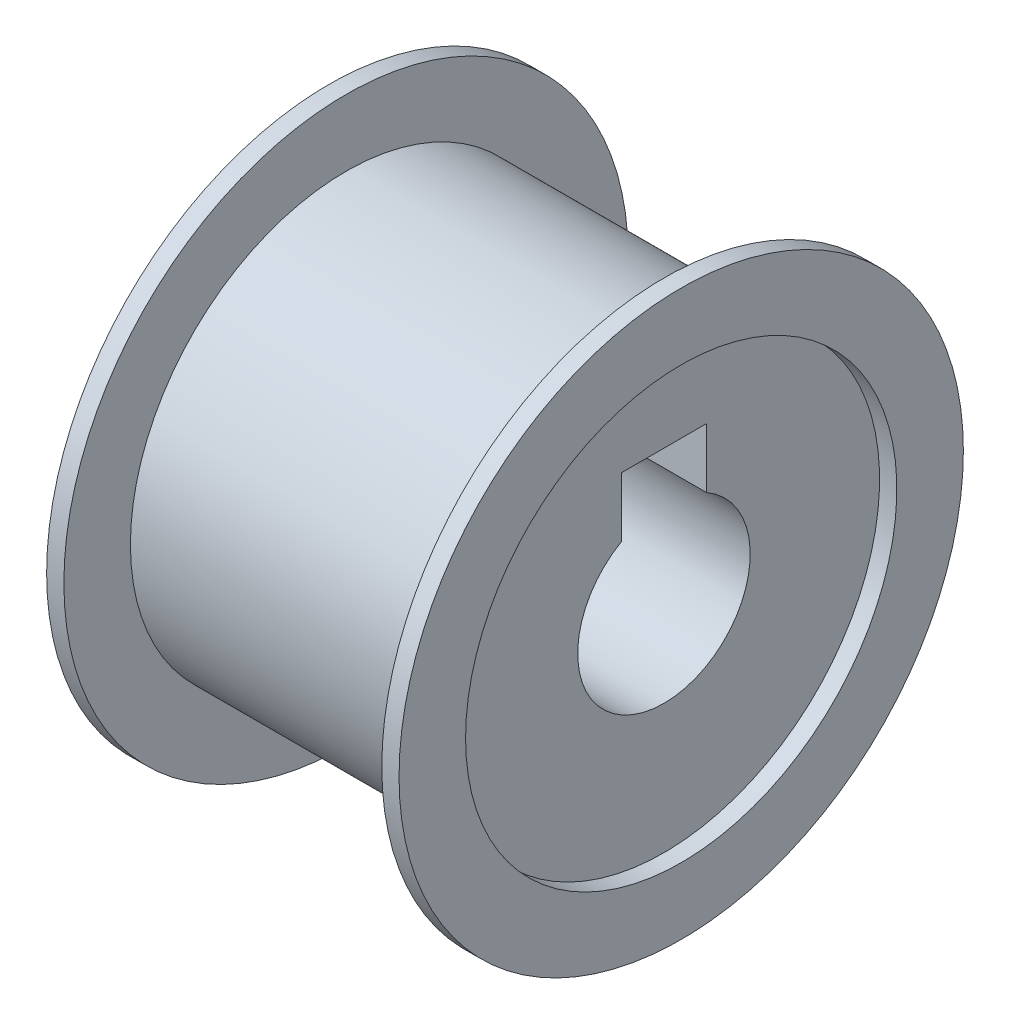
SolidWorks part; units mm, degrees
ref_plane "Front Plane" through (0, 0, 0) normal (0, 0, 1) x (1, 0, 0)
ref_plane "Top Plane" through (0, 0, 0) normal (0, 1, 0) x (1, 0, 0)
ref_plane "Right Plane" through (0, 0, 0) normal (1, 0, 0) x (0, 0, -1)
sketch "Sketch1" plane through (0, 0, 0) normal (0, 1, 0) x (1, 0, 0)
  line L0 (0, 0) -> (3.0534, 0) construction
  line L5 (-2.0429, 2.5) -> (2.0429, 2.5)
  line L6 (-2.0429, 2.5) -> (-2.0429, 1)
  line L15 (-2.0429, 1) -> (2.0429, 1)
  line L16 (2.0429, 2.5) -> (2.0429, 1)
  line L17 (-2.0429, 2.5) -> (2.0429, 1) construction
  line L18 (-2.0429, 1) -> (2.0429, 2.5) construction
  line L19 (2.0429, 1) -> (1.8429, 1)
  line L20 (2.0429, 1) -> (2.0429, 3.2714)
  line L21 (2.0429, 3.2714) -> (1.8429, 3.2714)
  line L22 (1.8429, 1) -> (1.8429, 3.2714)
  line L23 (-2.0429, 1) -> (-1.8429, 1)
  line L24 (-2.0429, 1) -> (-2.0429, 3.2714)
  line L25 (-2.0429, 3.2714) -> (-1.8429, 3.2714)
  line L26 (-1.8429, 1) -> (-1.8429, 3.2714)
  point P0 (0, 1.75)
  dimension "D1" = 1
  dimension "D2" = 0.2
  dimension "D3" = 2.5
revolve "Revolve1" add sketch "Sketch1" angle 360 about L0
sketch "Sketch2" plane through (-1.8429, 0, 0) normal (-1, 0, 0) x (0, 0, 1)
  line L0 (0.4947, 0.2083) -> (-0.4947, 0.2083)
  line L1 (-0.4947, -1.5622) -> (0.4947, -1.5622)
  line L2 (-0.4947, -1.5622) -> (-0.4947, 1.5622)
  line L3 (-0.4947, 1.5622) -> (0.4947, 1.5622)
  line L4 (0.4947, -1.5622) -> (0.4947, 1.5622)
  line L5 (-0.4947, -1.5622) -> (0.4947, 1.5622) construction
  line L6 (-0.4947, 1.5622) -> (0.4947, -1.5622) construction
  point P0 (0, 0)
  circle M6 centre (0, 0) radius 1
  dimension "D1" = 1.5622
extrude "Cut-Extrude1" cut sketch "Sketch2" against normal blind 10 contours L4 L3 L2 M6
